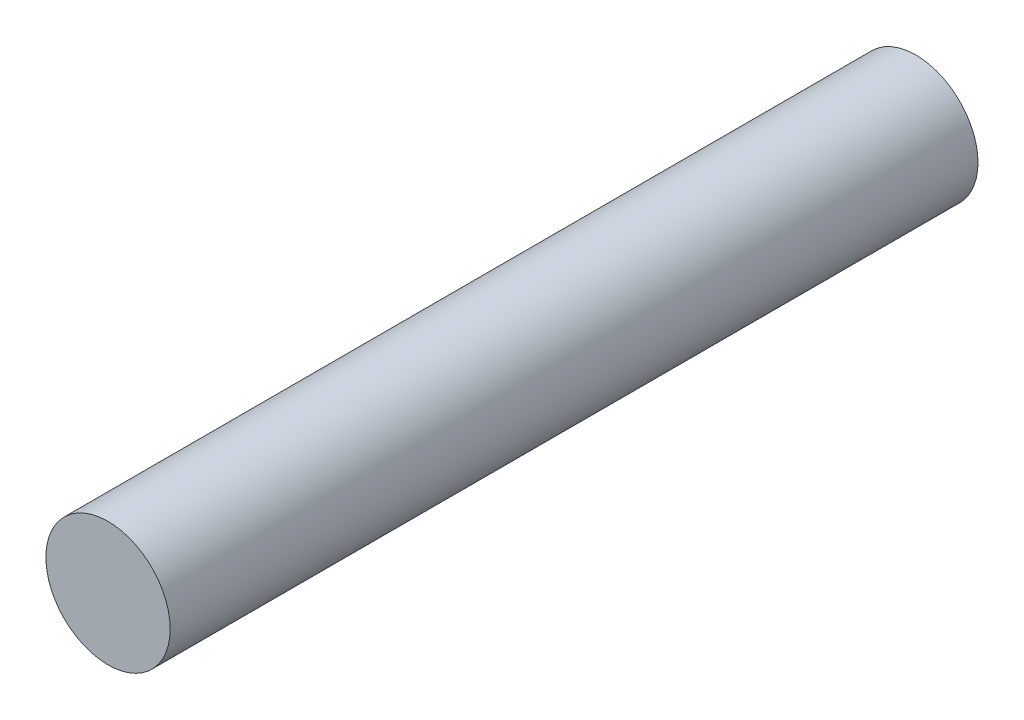
from build123d import *

# Parameters (mm, degrees)
SKETCH_1_R      = 10
EXTRUDE_1_DEPTH = 130


with BuildPart() as part:
    # 草图1 → 凸台-拉伸1 (new body)
    with BuildSketch(Plane.XY):
        Circle(SKETCH_1_R)
    extrude(amount=EXTRUDE_1_DEPTH)


solid = part.part
